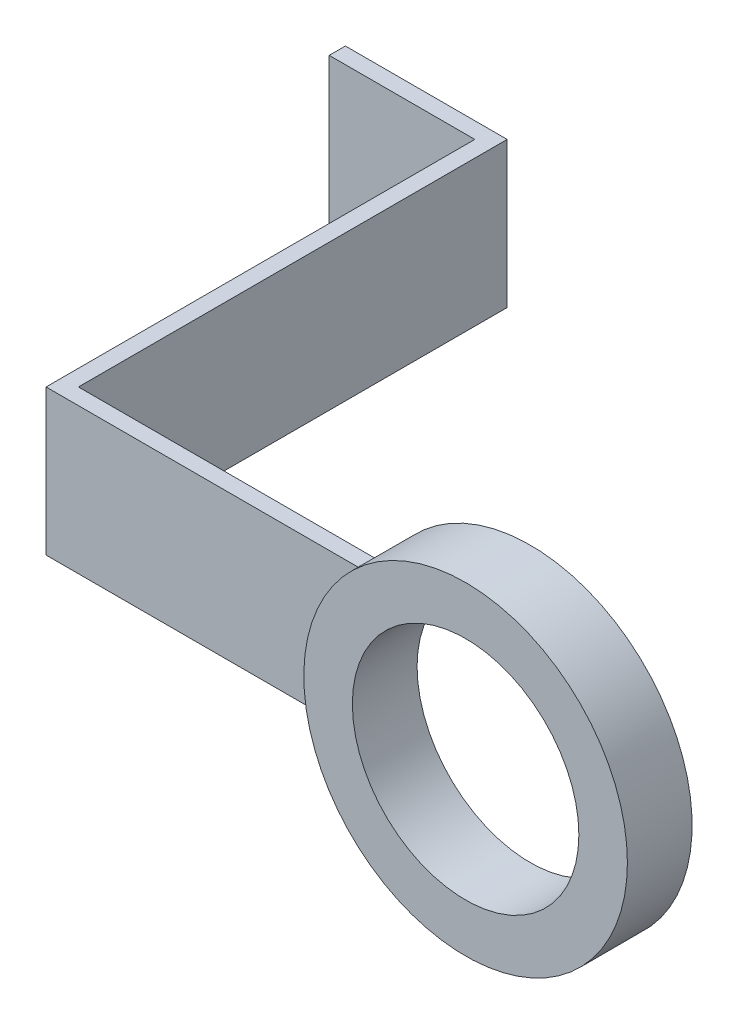
SolidWorks part; units mm, degrees
ref_plane "前视基准面" through (0, 0, 0) normal (0, 0, 1) x (1, 0, 0)
ref_plane "上视基准面" through (0, 0, 0) normal (0, 1, 0) x (1, 0, 0)
ref_plane "右视基准面" through (0, 0, 0) normal (1, 0, 0) x (0, 0, -1)
sketch "草图1" plane through (0, 0, 0) normal (0, 0, 1) x (1, 0, 0)
  circle A0 centre (0, 0) radius 14
  circle A1 centre (0, 0) radius 20
  dimension "D1" = 28
  dimension "D2" = 40
extrude "凸台-拉伸1" add sketch "草图1" along normal mid plane 8
sketch "草图2" plane through (0, 0, -4) normal (0, 0, -1) x (-1, 0, 0)
  line L0 (17.8606, 9) -> (17.8606, -9)
  line L1 (17.8606, 9) -> (57.8606, 9)
  line L2 (57.8606, 9) -> (57.8606, -9)
  line L3 (57.8606, -9) -> (17.8606, -9)
  circle A0 centre (0, 0) radius 20 construction
  dimension "D1" = 18
  dimension "D2" = 40
extrude "凸台-拉伸2" add sketch "草图2" against normal blind 2
sketch "草图3" plane through (0, 0, -4) normal (0, 0, -1) x (-1, 0, 0)
  line L0 (17.8606, -9) -> (57.8606, -9) construction
  line L1 (57.8606, 9) -> (55.8606, 9)
  line L2 (57.8606, 9) -> (57.8606, -9)
  line L3 (57.8606, -9) -> (55.8606, -9)
  line L4 (55.8606, 9) -> (55.8606, -9)
  dimension "D1" = 2
extrude "凸台-拉伸3" add sketch "草图3" along normal blind 53
sketch "草图4" plane through (-57.8606, 0, 0) normal (-1, 0, 0) x (0, 0, 1)
  line L0 (-2, -9) -> (-57, -9) construction
  line L1 (-57, 9) -> (-55, 9)
  line L2 (-57, 9) -> (-57, -9)
  line L3 (-57, -9) -> (-55, -9)
  line L4 (-55, 9) -> (-55, -9)
  dimension "D1" = 2
extrude "凸台-拉伸4" add sketch "草图4" along normal blind 18
